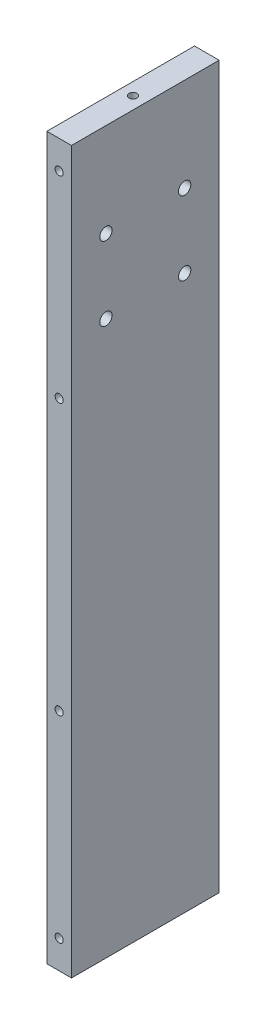
from build123d import *

# Parameters (mm, degrees)
SKETCH1_W                  = 10
SKETCH1_H                  = 293
BOSS_EXTRUDE1_DEPTH        = 30
M4_TAPPED_HOLE1_AT_2_COUNT = 2
M4_TAPPED_HOLE1_AT_2_PITCH = 270
M4_TAPPED_HOLE1_AT_3_COUNT = 2
M4_TAPPED_HOLE1_AT_3_PITCH = 80
M4_TAPPED_HOLE1_AT_4_COUNT = 2
M4_TAPPED_HOLE1_AT_4_PITCH = 190
M6_TAPPED_HOLE1_D          = 5


with BuildPart() as part:
    # Sketch1 → Boss-Extrude1 (new, symmetric)
    with BuildSketch(Plane.XY):
        Rectangle(SKETCH1_W, SKETCH1_H)
    extrude(amount=BOSS_EXTRUDE1_DEPTH, both=True)

    # Sketch4 → M4 Tapped Hole1 (revolve, cut)
    with BuildSketch(Plane(origin=(0, 135, 30), x_dir=(0, -1, 0), z_dir=(1, 0, 0))):
        Polygon((0, 0), (0, 12.491420021), (1.65, 11.5), (1.65, 0), align=None)
    m4_tapped_hole1 = revolve(axis=Axis((0, 135, 36.35), (0, 0, -1)), mode=Mode.SUBTRACT)

    # M4 Tapped Hole1 at 2: M4 Tapped Hole1 ×2
    with Locations(*[(0, -i * M4_TAPPED_HOLE1_AT_2_PITCH, 0) for i in range(1, M4_TAPPED_HOLE1_AT_2_COUNT)]):
        add(m4_tapped_hole1, mode=Mode.SUBTRACT)

    # M4 Tapped Hole1 at 3: M4 Tapped Hole1 ×2
    with Locations(*[(0, -i * M4_TAPPED_HOLE1_AT_3_PITCH, 0) for i in range(1, M4_TAPPED_HOLE1_AT_3_COUNT)]):
        add(m4_tapped_hole1, mode=Mode.SUBTRACT)

    # M4 Tapped Hole1 at 4: M4 Tapped Hole1 ×2
    with Locations(*[(0, -i * M4_TAPPED_HOLE1_AT_4_PITCH, 0) for i in range(1, M4_TAPPED_HOLE1_AT_4_COUNT)]):
        add(m4_tapped_hole1, mode=Mode.SUBTRACT)

    # Sketch6 → M4 Tapped Hole2 (revolve, cut)
    with BuildSketch(Plane(origin=(0, -146.5, 0), x_dir=(0, 0, -1), z_dir=(1, 0, 0))):
        Polygon((0, 0), (0, 12.491420021), (1.65, 11.5), (1.65, 0), align=None)
    m4_tapped_hole2 = revolve(axis=Axis((0, -152.85, 0), (0, 1, 0)), mode=Mode.SUBTRACT)

    # Mirror1: M4 Tapped Hole2 across plane
    add(m4_tapped_hole2.mirror(Plane.ZX), mode=Mode.SUBTRACT)

    # M6 Tapped Hole1 (through all)
    with Locations(Plane(origin=(5, 0, 0), x_dir=(0, 0, -1), z_dir=(1, 0, 0))):
        with Locations((-16, 78.5), (16, 78.5), (16, 108.5), (-16, 108.5)):
            Hole(M6_TAPPED_HOLE1_D / 2)

    # Mirror2: M4 Tapped Hole1 across plane
    add(m4_tapped_hole1.mirror(Plane.XY), mode=Mode.SUBTRACT)

    # Mirror2 copy 1 sketch → Mirror2 copy 1 (revolve, cut)
    with BuildSketch(Plane(origin=(0, -135, -30), x_dir=(0, -1, 0), z_dir=(1, 0, 0))):
        Polygon((0, 0), (0, -12.491420021), (1.65, -11.5), (1.65, 0), align=None)
    revolve(axis=Axis((0, -135, -36.35), (0, 0, -1)), mode=Mode.SUBTRACT)

    # Mirror2 copy 2 sketch → Mirror2 copy 2 (revolve, cut)
    with BuildSketch(Plane(origin=(0, 55, -30), x_dir=(0, -1, 0), z_dir=(1, 0, 0))):
        Polygon((0, 0), (0, -12.491420021), (1.65, -11.5), (1.65, 0), align=None)
    revolve(axis=Axis((0, 55, -36.35), (0, 0, -1)), mode=Mode.SUBTRACT)

    # Mirror2 copy 3 sketch → Mirror2 copy 3 (revolve, cut)
    with BuildSketch(Plane(origin=(0, -55, -30), x_dir=(0, -1, 0), z_dir=(1, 0, 0))):
        Polygon((0, 0), (0, -12.491420021), (1.65, -11.5), (1.65, 0), align=None)
    revolve(axis=Axis((0, -55, -36.35), (0, 0, -1)), mode=Mode.SUBTRACT)


solid = part.part
